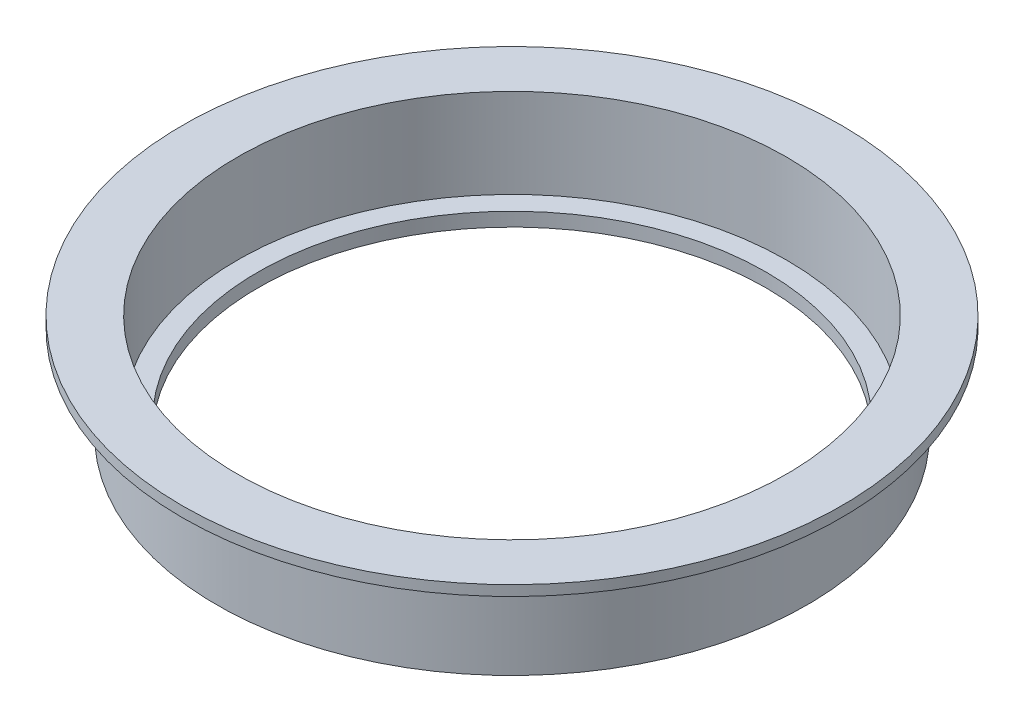
SolidWorks part; units mm, degrees
ref_plane "前视基准面" through (0, 0, 0) normal (0, 0, 1) x (1, 0, 0)
ref_plane "上视基准面" through (0, 0, 0) normal (0, 1, 0) x (1, 0, 0)
ref_plane "右视基准面" through (0, 0, 0) normal (1, 0, 0) x (0, 0, -1)
sketch "草图1" plane through (0, 0, 0) normal (0, 0, 1) x (1, 0, 0)
  line L0 (-37, 0) -> (-37, 2)
  line L1 (-37, 2) -> (-40, 2)
  line L2 (-40, 2) -> (-40, 15)
  line L3 (-40, 15) -> (-48, 15)
  line L4 (-48, 15) -> (-48, 13.5)
  line L5 (-48, 13.5) -> (-43, 13.5)
  line L6 (-43, 13.5) -> (-43, 0)
  line L7 (-43, 0) -> (-37, 0)
  line L8 (0, 0) -> (0, 18.7449) construction
  dimension "D1" = 74
  dimension "D2" = 43
  dimension "D3" = 80
  dimension "D4" = 15
  dimension "D5" = 1.5
  dimension "D6" = 2
  dimension "D7" = 8
revolve "旋转1" add sketch "草图1" angle 360 about L8
equation "\"图号代码1\"= \"图号代码\""
equation "\"名称代码2\"= \"名称代码\""
